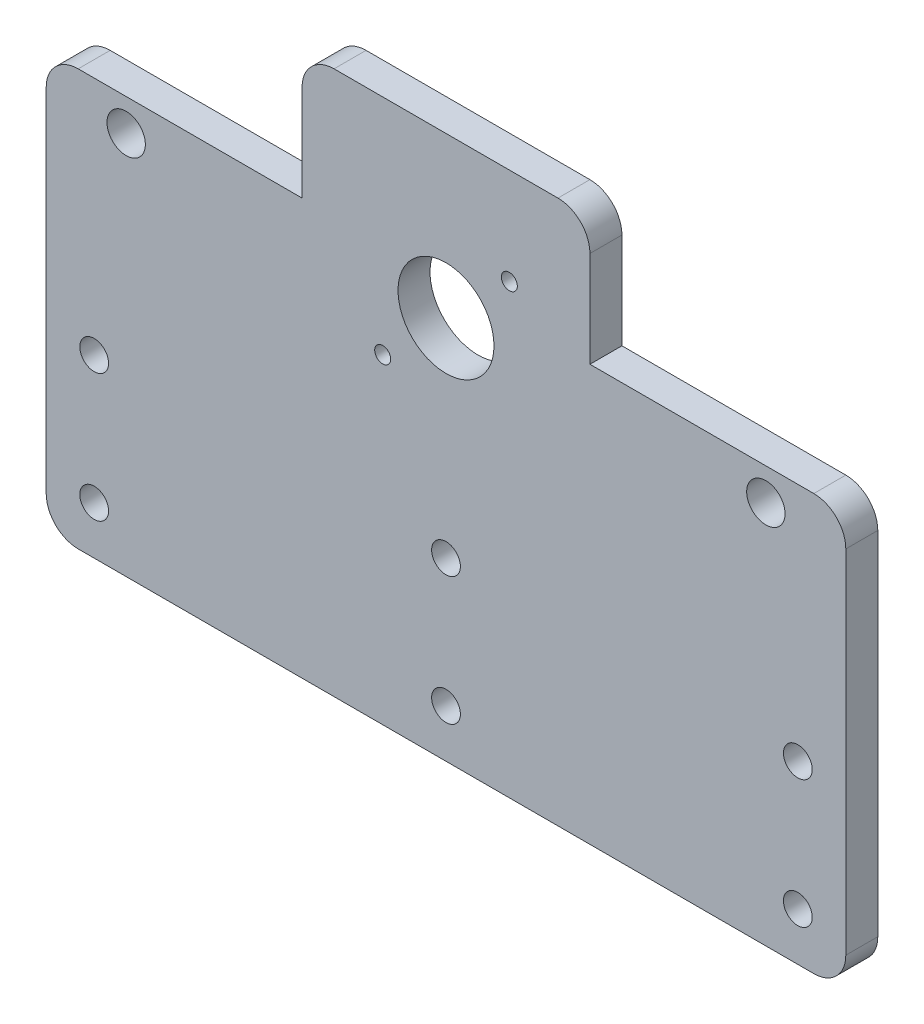
from build123d import *

# Parameters (mm, degrees)
SKETCH_1_W              = 250
SKETCH_1_H              = 170
EXTRUDE_1_DEPTH         = 5
SKETCH_2_W              = 80
SKETCH_2_H              = 40
CUT_EXTRUDE_1_DEPTH     = 10
HOLE_WIZARD_9_0_9_1_D   = 9
PATTERN_LINEAR_1_COUNT  = 3
PATTERN_LINEAR_1_PITCH  = 110
HOLE_WIZARD_12_0_12_1_D = 12
SKETCH_7_R              = 15
CUT_EXTRUDE_2_DEPTH     = 10
HOLE_WIZARD_M6_1_D      = 5
FILLET_1_R              = 10


with BuildPart() as part:
    # 草图1 → 凸台-拉伸1 (new, symmetric)
    with BuildSketch(Plane.XY):
        Rectangle(SKETCH_1_W, SKETCH_1_H)
    extrude(amount=EXTRUDE_1_DEPTH, both=True)

    # 草图2 → 切除-拉伸1 (cut)
    with BuildSketch(Plane.XY.offset(5)):
        with Locations((85, 65)):
            Rectangle(SKETCH_2_W, SKETCH_2_H)
    cut_extrude_1 = extrude(amount=-CUT_EXTRUDE_1_DEPTH, mode=Mode.SUBTRACT)

    # 镜向1: 切除-拉伸1 across plane
    add(cut_extrude_1.mirror(Plane(origin=(0, 0, 0), x_dir=(0, 0, 1), z_dir=(1, 0, 0))), mode=Mode.SUBTRACT)

    # Ø9.0 (9) 直径孔1 (through all)
    with Locations(Plane.XY.offset(5)):
        with Locations((-110, -30), (-110, -70)):
            hole_wizard_9_0_9_1 = Hole(HOLE_WIZARD_9_0_9_1_D / 2)

    # 阵列(线性)1: Ø9.0 (9) 直径孔1 ×3
    with Locations(*[(i * PATTERN_LINEAR_1_PITCH, 0, 0) for i in range(1, PATTERN_LINEAR_1_COUNT)]):
        add(hole_wizard_9_0_9_1, mode=Mode.SUBTRACT)

    # Ø12.0 (12) 直径孔1 (through all)
    with Locations(Plane.XY.offset(5)):
        with Locations((-100, 35), (100, 35)):
            Hole(HOLE_WIZARD_12_0_12_1_D / 2)

    # 草图7 → 切除-拉伸2 (cut)
    with BuildSketch(Plane.XY.offset(5)):
        with Locations((0, 35)):
            Circle(SKETCH_7_R)
    extrude(amount=-CUT_EXTRUDE_2_DEPTH, mode=Mode.SUBTRACT)

    # M6 螺纹孔1 (through all)
    with Locations(Plane.XY.offset(5)):
        with Locations((-19.8, 15.2), (19.8, 54.8)):
            Hole(HOLE_WIZARD_M6_1_D / 2)

    # 圆角1
    fillet_1_edges = [part.edges().sort_by_distance(p)[0] for p in [
        (45, 85, 0),
        (125, 45, 0),
        (-45, 85, 0),
        (-125, 45, 0),
        (125, -85, 0),
        (-125, -85, 0),
    ]]
    fillet(fillet_1_edges, radius=FILLET_1_R)


solid = part.part
